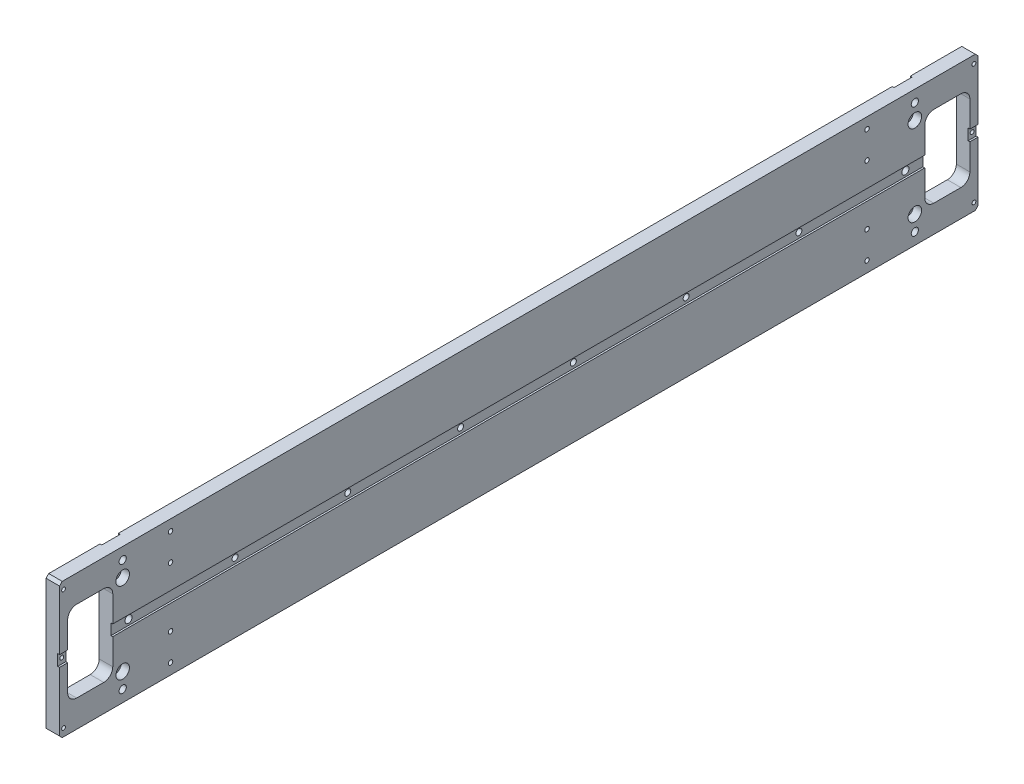
SolidWorks part; units mm, degrees
material "6061 合金"
ref_plane "前视基准面" through (0, 0, 0) normal (0, 0, 1) x (1, 0, 0)
ref_plane "上视基准面" through (0, 0, 0) normal (0, 1, 0) x (1, 0, 0)
ref_plane "右视基准面" through (0, 0, 0) normal (1, 0, 0) x (0, 0, -1)
sketch "草图1" plane through (0, 0, 0) normal (1, 0, 0) x (0, 0, -1)
  line L2 (-509, 75) -> (509, -75) construction
  line L3 (509, 75) -> (-509, -75) construction
  line L5 (-509, 75) -> (509, 75)
  line L6 (-509, 75) -> (-509, -75)
  line L7 (-509, -75) -> (509, -75)
  line L8 (509, 75) -> (509, -75)
  dimension "D1" = 1018
  dimension "D3" = 150
extrude "凸台-拉伸1" add sketch "草图1" along normal blind 15 contours L7 L8 L5 L6
sketch "草图2" plane through (15, 0, 0) normal (1, 0, 0) x (0, 0, -1)
  line L1 (-706.1007, 6.1) -> (706.1007, 6.1)
  line L2 (-706.1007, 6.1) -> (-706.1007, -6.1)
  line L3 (-706.1007, -6.1) -> (706.1007, -6.1)
  line L4 (706.1007, 6.1) -> (706.1007, -6.1)
  line L5 (-706.1007, 6.1) -> (706.1007, -6.1) construction
  line L6 (-706.1007, -6.1) -> (706.1007, 6.1) construction
  point P0 (0, 0)
  dimension "D1" = 0
  dimension "D2" = 12.2
extrude "切除-拉伸1" cut sketch "草图2" against normal blind 2
sketch "草图15" plane through (0, 0, 0) normal (-1, 0, 0) x (0, 0, 1)
  line L0 (-509, 75) -> (-509, -75) construction
  line L1 (-428.9, -280.207) -> (-449.1, -280.207)
  line L2 (-428.9, -280.207) -> (-428.9, 251.8468)
  line L3 (-428.9, 251.8468) -> (-449.1, 251.8468)
  line L4 (-449.1, -280.207) -> (-449.1, 251.8468)
  line L5 (-428.9, -280.207) -> (-449.1, 251.8468) construction
  line L6 (-428.9, 251.8468) -> (-449.1, -280.207) construction
  line L7 (449.1, -328.3233) -> (428.9, -328.3233)
  line L8 (449.1, -328.3233) -> (449.1, 283.9426)
  line L9 (449.1, 283.9426) -> (428.9, 283.9426)
  line L10 (428.9, -328.3233) -> (428.9, 283.9426)
  line L11 (449.1, -328.3233) -> (428.9, 283.9426) construction
  line L12 (449.1, 283.9426) -> (428.9, -328.3233) construction
  line L13 (509, 75) -> (509, -75) construction
  point P0 (-439, -14.1801)
  point P5 (439, -22.1904)
  dimension "D1" = 20.2
  dimension "D2" = 70
  dimension "D3" = 70
  dimension "D4" = 20.2
extrude "切除-拉伸4" cut sketch "草图15" against normal blind 2
chamfer "倒角1" distance 3 angle 45 4 edges at (7.5, 75, -509) (7.5, -75, -509) (7.5, 75, 509) (7.5, -75, 509)
sketch "草图24" plane through (15, 0, 0) normal (1, 0, 0) x (0, 0, -1)
  line L1 (-500, 45) -> (-450, 45)
  line L2 (-500, 45) -> (-500, -45)
  line L3 (-500, -45) -> (-450, -45)
  line L4 (-450, 45) -> (-450, -45)
  line L5 (-500, 45) -> (-450, -45) construction
  line L6 (-500, -45) -> (-450, 45) construction
  line L8 (-509, 72) -> (-509, 6.1) construction
  point P0 (-475, 0)
  dimension "D1" = 9
  dimension "D2" = 50
  dimension "D4" = 90
extrude "切除-拉伸5" cut sketch "草图24" against normal through all
fillet "圆角2" radius 10 4 edges at (7.5, -45, 450) (7.5, -45, 500) (7.5, 45, 450) (7.5, 45, 500)
mirror "镜向1" about plane through (0, 0, 0) normal (0, 0, 1) of "圆角2", "切除-拉伸5"
hole_wizard "打孔尺寸(%根据)开槽圆柱头螺钉的类型9" positions "草图30" profile "草图32" counterbore size "M8" standard "GB" end condition through all
sketch "草图30" plane through (15, 0, 0) normal (1, 0, 0) x (0, 0, -1)
  point P0 (439, 45)
  point P6 (439, -45)
sketch "草图32" plane through (15, 45, -439) normal (0, 1, 0) x (0, 0, -1)
  line L0 (0, 0) -> (0, 15)
  line L1 (0, 15) -> (4.5, 15)
  line L3 (4.5, 15) -> (4.5, 9)
  line L4 (4.5, 9) -> (7.5, 9)
  line L5 (7.5, 9) -> (7.5, 0)
  line L7 (7.5, 0) -> (0, 0)
  line L11 (0, -6.35) -> (0, 107.95) construction
  dimension "通孔孔直径" = 9
  dimension "通孔孔深度" = 15
  dimension "柱形沉头孔直径" = 15
  dimension "柱形沉头孔深度" = 9
hole_wizard "大小mm 暗销孔2" positions "草图33" profile "草图34" hole size "Ø8.0" standard "GB"
sketch "草图33" plane through (15, 0, 0) normal (1, 0, 0) x (0, 0, -1)
  line L0 (439, 0) -> (483.2381, 0) construction
  line L1 (-506, -75) -> (506, -75) construction
  line L2 (-506, 75) -> (506, 75) construction
  point P0 (439, 62)
  point P15 (439, -62)
sketch "草图34" plane through (15, 62, -439) normal (0, 1, 0) x (0, 0, -1)
  line L0 (0, 0) -> (0, 17.4034)
  line L1 (0, 17.4034) -> (4, 15)
  line L2 (4, 15) -> (4, 0)
  line L5 (4, 0) -> (0, 0)
  line L10 (0, 17.4034) -> (-4, 15) construction
  line L11 (0, -6.35) -> (0, 107.95) construction
  dimension "孔直径" = 8
  dimension "孔深度" = 15
  dimension "导头角度" = 118
hole_wizard "M6 螺纹孔1" positions "草图35" profile "草图36" tap size "M6" standard "GB" end condition through all
sketch "草图35" plane through (0, 0, 0) normal (-1, 0, 0) x (0, 0, 1)
  point P0 (-386, 63)
  point P3 (-386, 33)
  point P6 (-386, -33)
  point P9 (-386, -63)
sketch "草图36" plane through (0, 63, -386) normal (0, 1, 0) x (0, 0, 1)
  line L0 (0, 0) -> (0, 15)
  line L1 (0, 15) -> (2.5, 15)
  line L2 (2.5, 15) -> (2.5, 0)
  line L5 (2.5, 0) -> (0, 0)
  line L11 (0, -6.35) -> (0, 107.95) construction
  dimension "通孔螺纹孔钻头直径" = 5
  dimension "通孔螺纹孔钻头深度" = 15
cosmetic thread "孔螺蚊线36" parameters "D2"=6
cosmetic thread "孔螺蚊线37" parameters "D2"=6
cosmetic thread "孔螺蚊线38" parameters "D2"=6
cosmetic thread "孔螺蚊线39" parameters "D2"=6
ref_plane "基准面1" through (0, 0, 0) normal (0, 0, -1) x (-1, 0, 0)
hole_wizard "打孔尺寸(%根据)开槽圆柱头螺钉的类型9" positions "草图37" profile "草图38" counterbore size "M6" standard "GB" end condition through all
sketch "草图37" plane through (0, 0, 0) normal (-1, 0, 0) x (0, 0, 1)
  point P0 (-312.5, 0)
  point P3 (-187.5, 0)
  point P6 (-62.5, 0)
  point P9 (62.5, 0)
  point P12 (187.5, 0)
  point P15 (312.5, 0)
sketch "草图38" plane through (0, 0, -312.5) normal (0, 1, 0) x (0, 0, 1)
  line L0 (0, 0) -> (0, 15)
  line L1 (0, 15) -> (3.3, 15)
  line L3 (3.3, 15) -> (3.3, 6.8)
  line L4 (3.3, 6.8) -> (5.5, 6.8)
  line L5 (5.5, 6.8) -> (5.5, 0)
  line L7 (5.5, 0) -> (0, 0)
  line L11 (0, -6.35) -> (0, 107.95) construction
  dimension "通孔孔直径" = 6.6
  dimension "通孔孔深度" = 15
  dimension "柱形沉头孔直径" = 11
  dimension "柱形沉头孔深度" = 6.8
hole_wizard "大小mm 暗销孔3" positions "草图39" profile "草图40" hole size "Ø8.0" standard "GB" end condition through all
sketch "草图39" plane through (0, 0, 0) normal (-1, 0, 0) x (0, 0, 1)
  point P0 (430.5, 0)
  point P3 (-430.5, 0)
sketch "草图40" plane through (0, 0, 430.5) normal (0, 1, 0) x (0, 0, 1)
  line L0 (0, 0) -> (0, 15)
  line L1 (0, 15) -> (4, 15)
  line L2 (4, 15) -> (4, 0)
  line L5 (4, 0) -> (0, 0)
  line L11 (0, -6.35) -> (0, 107.95) construction
  dimension "通孔孔直径" = 8
  dimension "通孔孔深度" = 15
hole_wizard "打孔尺寸(%根据)内六角圆柱头螺钉的类型0" positions "草图41" profile "草图42" counterbore size "M4" standard "GB" end condition through all
sketch "草图41" plane through (0, 0, 0) normal (-1, 0, 0) x (0, 0, 1)
  circle A0 centre (-504.5, 0) radius 1.65 construction
  point P0 (-504.5, 66.5)
  point P3 (-504.5, 0)
  point P6 (-504.5, -66.5)
  point P10 (0, 0)
  point P11 (-485.147, -6.3199)
  point P12 (0, 0)
  point P15 (0, 0)
sketch "草图42" plane through (0, 66.5, -504.5) normal (0, 1, 0) x (0, 0, 1)
  line L0 (0, 0) -> (0, 15)
  line L1 (0, 15) -> (2.15, 15)
  line L3 (2.15, 15) -> (2.15, 5)
  line L4 (2.15, 5) -> (4, 5)
  line L5 (4, 5) -> (4, 0)
  line L7 (4, 0) -> (0, 0)
  line L11 (0, -6.35) -> (0, 107.95) construction
  dimension "通孔孔直径" = 4.3
  dimension "通孔孔深度" = 15
  dimension "柱形沉头孔直径" = 8
  dimension "柱形沉头孔深度" = 5
mirror "镜向2" about plane through (0, 0, 0) normal (0, 0, 1) of "M6 螺纹孔1", "大小mm 暗销孔2", "打孔尺寸(%根据)开槽圆柱头螺钉的类型9", "大小mm 暗销孔3", "打孔尺寸(%根据)内六角圆柱头螺钉的类型0"
